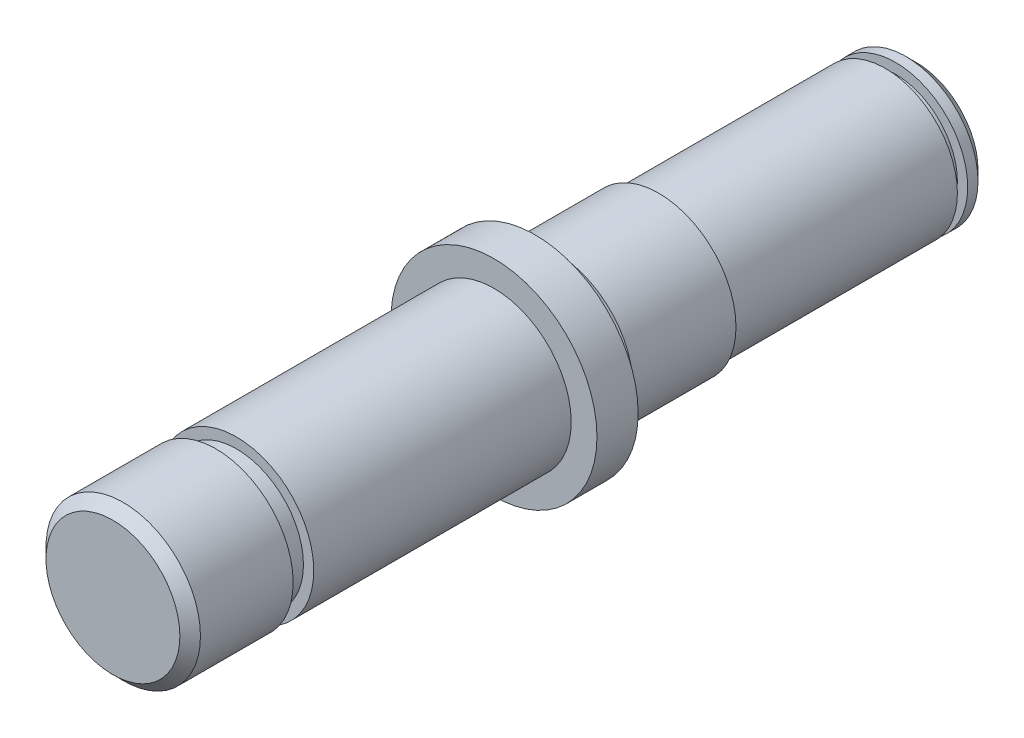
from build123d import *

# Parameters (mm, degrees)
SKETCH2_R           = 7
BOSS_EXTRUDE1_DEPTH = 2
SKETCH3_R           = 6
BOSS_EXTRUDE2_DEPTH = 1
SKETCH4_R           = 7
BOSS_EXTRUDE3_DEPTH = 22
SKETCH5_R           = 7.5
BOSS_EXTRUDE4_DEPTH = 10
SKETCH6_R           = 6.5
BOSS_EXTRUDE5_DEPTH = 2
SKETCH7_R           = 10
BOSS_EXTRUDE6_DEPTH = 4
SKETCH8_R           = 7.5
BOSS_EXTRUDE7_DEPTH = 25
SKETCH9_R           = 6.5
BOSS_EXTRUDE8_DEPTH = 2
SKETCH10_R          = 7.5
BOSS_EXTRUDE9_DEPTH = 10
CHAMFER1_SIZE       = 1
CUT_EXTRUDE1_START  = -4
CUT_EXTRUDE1_DEPTH  = 10
CUT_EXTRUDE2_START  = -4.5
CUT_EXTRUDE2_DEPTH  = 10


with BuildPart() as part:
    # Sketch2 → Boss-Extrude1 (new body)
    with BuildSketch(Plane.XY):
        Circle(SKETCH2_R)
    extrude(amount=BOSS_EXTRUDE1_DEPTH)

    # Sketch3 → Boss-Extrude2 (add)
    with BuildSketch(Plane.XY.offset(2)):
        Circle(SKETCH3_R)
    extrude(amount=BOSS_EXTRUDE2_DEPTH)

    # Sketch4 → Boss-Extrude3 (add)
    with BuildSketch(Plane.XY.offset(3)):
        Circle(SKETCH4_R)
    extrude(amount=BOSS_EXTRUDE3_DEPTH)

    # Sketch5 → Boss-Extrude4 (add)
    with BuildSketch(Plane.XY.offset(25)):
        Circle(SKETCH5_R)
    extrude(amount=BOSS_EXTRUDE4_DEPTH)

    # Sketch6 → Boss-Extrude5 (add)
    with BuildSketch(Plane.XY.offset(35)):
        Circle(SKETCH6_R)
    extrude(amount=BOSS_EXTRUDE5_DEPTH)

    # Sketch7 → Boss-Extrude6 (add)
    with BuildSketch(Plane.XY.offset(37)):
        Circle(SKETCH7_R)
    extrude(amount=BOSS_EXTRUDE6_DEPTH)

    # Sketch8 → Boss-Extrude7 (add)
    with BuildSketch(Plane.XY.offset(41)):
        Circle(SKETCH8_R)
    extrude(amount=BOSS_EXTRUDE7_DEPTH)

    # Sketch9 → Boss-Extrude8 (add)
    with BuildSketch(Plane.XY.offset(66)):
        Circle(SKETCH9_R)
    extrude(amount=BOSS_EXTRUDE8_DEPTH)

    # Sketch10 → Boss-Extrude9 (add)
    with BuildSketch(Plane.XY.offset(68)):
        Circle(SKETCH10_R)
    extrude(amount=BOSS_EXTRUDE9_DEPTH)

    # Chamfer1
    chamfer1_edges = [part.edges().sort_by_distance(p)[0] for p in [
        (-7, 0, 0),
        (-7.5, 0, 78),
    ]]
    chamfer(chamfer1_edges, length=CHAMFER1_SIZE)

    # Sketch11 → Cut-Extrude1 (cut)
    with BuildSketch(Plane(origin=(0, 0, 0), x_dir=(1, 0, 0), z_dir=(0, 1, 0)).offset(CUT_EXTRUDE1_START)):
        with BuildLine():
            ThreePointArc((2.5, -6.5), (1.767766953, -4.732233047), (0, -4))
            Line((0, -4), (0, -22))
            ThreePointArc((0, -22), (1.767766953, -21.267766953), (2.5, -19.5))
            Line((2.5, -19.5), (2.5, -6.5))
        make_face()
        with BuildLine():
            Line((0, -22), (0, -4))
            ThreePointArc((0, -4), (-1.767766953, -4.732233047), (-2.5, -6.5))
            Line((-2.5, -6.5), (-2.5, -19.5))
            ThreePointArc((-2.5, -19.5), (-1.767766953, -21.267766953), (0, -22))
        make_face()
    extrude(amount=-CUT_EXTRUDE1_DEPTH, mode=Mode.SUBTRACT)

    # Sketch12 → Cut-Extrude2 (cut)
    with BuildSketch(Plane(origin=(0, 0, 0), x_dir=(1, 0, 0), z_dir=(0, 1, 0)).offset(CUT_EXTRUDE2_START)):
        with BuildLine():
            Line((2.5, -45.5), (2.5, -58.5))
            ThreePointArc((2.5, -58.5), (0, -61), (-2.5, -58.5))
            Line((-2.5, -58.5), (-2.5, -45.5))
            ThreePointArc((-2.5, -45.5), (0, -43), (2.5, -45.5))
        make_face()
    extrude(amount=-CUT_EXTRUDE2_DEPTH, mode=Mode.SUBTRACT)


solid = part.part
